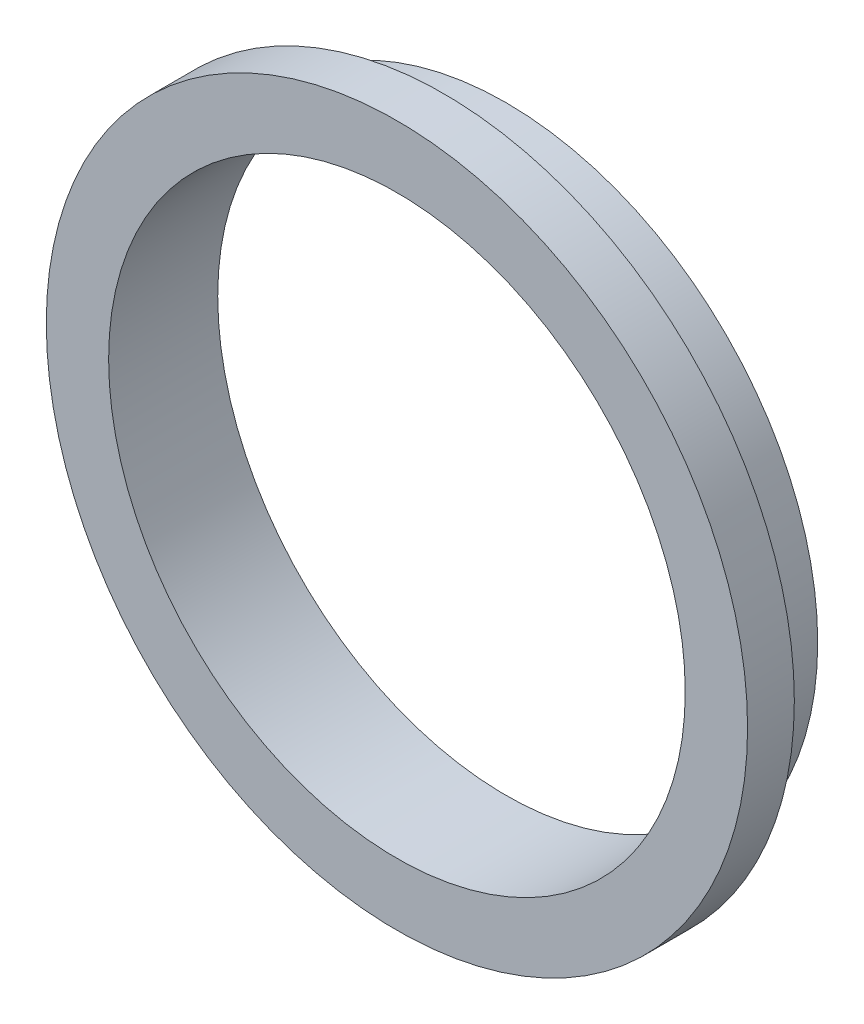
SolidWorks part; units mm, degrees
ref_plane "Front Plane" through (0, 0, 0) normal (0, 0, 1) x (1, 0, 0)
ref_plane "Top Plane" through (0, 0, 0) normal (0, 1, 0) x (1, 0, 0)
ref_plane "Right Plane" through (0, 0, 0) normal (1, 0, 0) x (0, 0, -1)
sketch "Sketch1" plane through (0, 0, 0) normal (0, 0, 1) x (1, 0, 0)
  circle A0 centre (0, 0) radius 22.5
  circle A1 centre (0, 0) radius 18.5
  dimension "D1" = 45
  dimension "D2" = 37
extrude "Boss-Extrude1" add sketch "Sketch1" along normal blind 3
sketch "Sketch3" plane through (0, 0, 0) normal (0, 0, -1) x (-1, 0, 0)
  circle A0 centre (0, 0) radius 20
  circle A1 centre (0, 0) radius 18.5
  dimension "D1" = 40
extrude "Boss-Extrude2" add sketch "Sketch3" along normal blind 4
